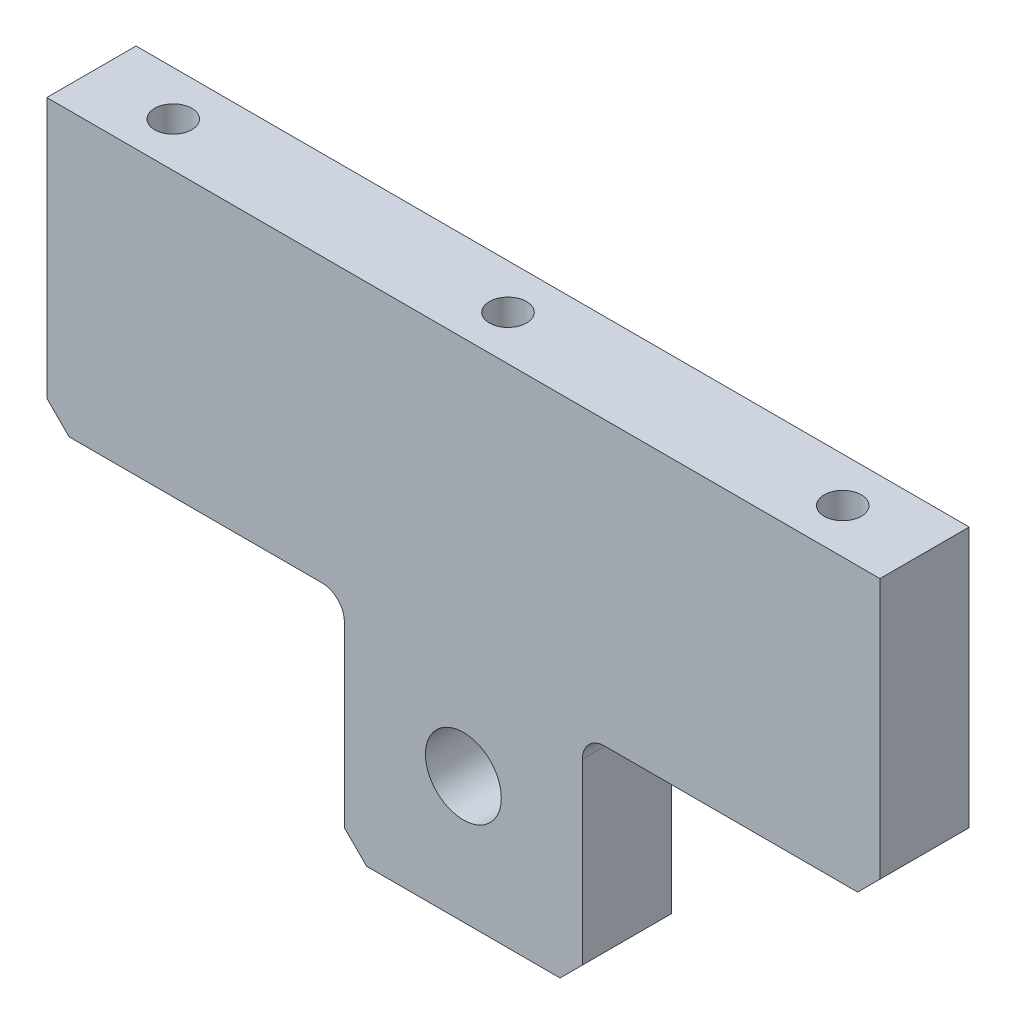
from build123d import *

# Parameters (mm, degrees)
SKETCH_1_W             = 112
SKETCH_1_H             = 68
EXTRUDE_1_DEPTH        = 12
SKETCH_2_W             = 40
SKETCH_2_H             = 30
CUT_EXTRUDE_1_DEPTH    = 12
HOLE_WIZARD_M12_1_D    = 10.2
CHAMFER_1_SIZE         = 3
FILLET_1_R             = 3
HOLE_WIZARD_M6_1_D     = 5
HOLE_WIZARD_M6_1_DEPTH = 15
HOLE_WIZARD_M6_1_TIP   = 1.502151548
HOLE_WIZARD_M5_1_D     = 4.2
HOLE_WIZARD_M5_1_DEPTH = 12.4
HOLE_WIZARD_M5_1_TIP   = 1.2618073


with BuildPart() as part:
    # 草图1 → 凸台-拉伸1 (new body)
    with BuildSketch(Plane.XY):
        with Locations((56, 34)):
            Rectangle(SKETCH_1_W, SKETCH_1_H)
    extrude(amount=EXTRUDE_1_DEPTH)

    # 草图2 → 切除-拉伸1 (cut)
    with BuildSketch(Plane.XY.offset(12)):
        with Locations((20, 15)):
            Rectangle(SKETCH_2_W, SKETCH_2_H)
    cut_extrude_1 = extrude(amount=-CUT_EXTRUDE_1_DEPTH, mode=Mode.SUBTRACT)

    # 镜向1: 切除-拉伸1 across plane
    add(cut_extrude_1.mirror(Plane.ZY.offset(-56)), mode=Mode.SUBTRACT)

    # M12 螺纹孔1 (through all)
    with Locations(Plane.XY.offset(12)):
        with Locations((56, 17)):
            Hole(HOLE_WIZARD_M12_1_D / 2)

    # 倒角1
    chamfer_1_edges = [part.edges().sort_by_distance(p)[0] for p in [
        (0, 30, 6),
        (40, 0, 6),
        (112, 30, 6),
        (72, 0, 6),
    ]]
    chamfer(chamfer_1_edges, length=CHAMFER_1_SIZE)

    # 圆角1
    fillet_1_edges = [part.edges().sort_by_distance(p)[0] for p in [
        (40, 30, 6),
        (72, 30, 6),
    ]]
    fillet(fillet_1_edges, radius=FILLET_1_R)

    # M6 螺纹孔1
    with Locations(Plane(origin=(0, 68, 0), x_dir=(1, 0, 0), z_dir=(0, 1, 0))):
        with Locations((101, -6), (56, -6), (11, -6)):
            Hole(HOLE_WIZARD_M6_1_D / 2, depth=HOLE_WIZARD_M6_1_DEPTH)
            with Locations((0, 0, -(HOLE_WIZARD_M6_1_DEPTH + HOLE_WIZARD_M6_1_TIP / 2))):  # 118° drill point
                Cone(0, HOLE_WIZARD_M6_1_D / 2, HOLE_WIZARD_M6_1_TIP, mode=Mode.SUBTRACT)

    # M5 螺纹孔1
    with Locations(Plane(origin=(0, 0, 0), x_dir=(-1, 0, 0), z_dir=(0, -1, 0))):
        with Locations((-63.5, -6), (-48.5, -6)):
            Hole(HOLE_WIZARD_M5_1_D / 2, depth=HOLE_WIZARD_M5_1_DEPTH)
            with Locations((0, 0, -(HOLE_WIZARD_M5_1_DEPTH + HOLE_WIZARD_M5_1_TIP / 2))):  # 118° drill point
                Cone(0, HOLE_WIZARD_M5_1_D / 2, HOLE_WIZARD_M5_1_TIP, mode=Mode.SUBTRACT)


solid = part.part
